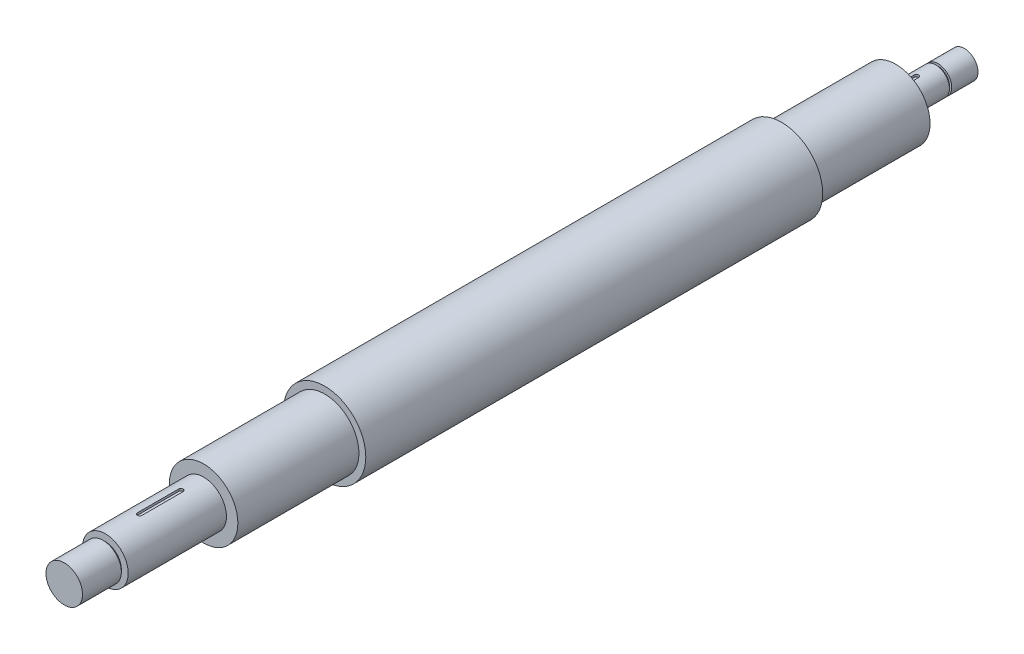
SolidWorks part; units mm, degrees
material "AISI 304"
ref_plane "Front Plane" through (0, 0, 0) normal (0, 0, 1) x (1, 0, 0)
ref_plane "Top Plane" through (0, 0, 0) normal (0, 1, 0) x (1, 0, 0)
ref_plane "Right Plane" through (0, 0, 0) normal (1, 0, 0) x (0, 0, -1)
sketch "Sketch1" plane through (0, 0, 0) normal (0, 0, 1) x (1, 0, 0)
  circle A0 centre (0, 0) radius 15
  dimension "D1" = 30
extrude "Boss-Extrude1" add sketch "Sketch1" along normal blind 50
sketch "Sketch2" plane through (0, 0, 50) normal (0, 0, 1) x (1, 0, 0)
  circle A0 centre (0, 0) radius 18
  dimension "D1" = 36
extrude "Boss-Extrude2" add sketch "Sketch2" along normal blind 200
sketch "Sketch3" plane through (0, 0, 250) normal (0, 0, 1) x (1, 0, 0)
  circle A0 centre (0, 0) radius 15
  dimension "D1" = 30
extrude "Boss-Extrude3" add sketch "Sketch3" along normal blind 53
sketch "Sketch4" plane through (0, 0, 0) normal (0, 0, -1) x (-1, 0, 0)
  circle A0 centre (0, 0) radius 6
  dimension "D1" = 12
extrude "Boss-Extrude4" add sketch "Sketch4" along normal blind 30
cosmetic thread "Cosmetic Thread1" parameters "D1"=11.4999, "D2"=11.5
sketch "Sketch5" plane through (0, 0, 0) normal (0, 1, 0) x (1, 0, 0)
  line L0 (0, 30) -> (0, -1.1912) construction
  line L1 (6, 30) -> (-6, 30) construction
  line L2 (15, 0) -> (-15, 0) construction
  line L3 (1, 9) -> (-1, 9)
  line L4 (1, 9) -> (1, 5)
  line L5 (1, 5) -> (-1, 5)
  line L6 (-1, 9) -> (-1, 5)
  line L7 (1, 9) -> (-1, 5) construction
  line L8 (1, 5) -> (-1, 9) construction
  circle A0 centre (0, 5) radius 1
  circle A1 centre (0, 9) radius 1
  point P7 (0, 7)
  point P16 (0, 5)
  dimension "D2" = 2
  dimension "D1" = 4
  dimension "D3" = 5
extrude "Cut-Extrude1" cut sketch "Sketch5" along normal blind 10 from offset 5 contours L3 A1 | L3 A1 | A1 L6 A0 L4 | L5 A0 | L5 A0
sketch "Sketch6" plane through (0, 0, -30) normal (0, 0, -1) x (-1, 0, 0)
  circle A0 centre (0, 0) radius 6
  circle A1 centre (0, 0) radius 5
  dimension "D1" = 10
extrude "Cut-Extrude3" cut sketch "Sketch6" against normal blind 1 from offset 11.5 offset against normal yes
sketch "Sketch7" plane through (0, 0, 303) normal (0, 0, 1) x (1, 0, 0)
  circle A0 centre (0, 0) radius 10
  dimension "D1" = 20
extrude "Boss-Extrude5" add sketch "Sketch7" along normal blind 43
sketch "Sketch9" plane through (0, 5, 0) normal (0, 1, 0) x (1, 0, 0)
  line L0 (0, -303) -> (0, -337.2251) construction
  line L1 (-10, -303) -> (10, -303) construction
  line L3 (-1, -313) -> (1, -313)
  line L4 (-1, -313) -> (-1, -331)
  line L5 (-1, -331) -> (1, -331)
  line L6 (1, -313) -> (1, -331)
  line L7 (-1, -313) -> (1, -331) construction
  line L8 (-1, -331) -> (1, -313) construction
  circle A0 centre (0, -313) radius 1
  circle A1 centre (0, -331) radius 1
  point P5 (0, -322)
  dimension "D1" = 2
  dimension "D2" = 18
  dimension "D3" = 10
extrude "Cut-Extrude4" cut sketch "Sketch9" along normal blind 12 from offset 4 contours A1 L6 A0 L4 | L5 A1 | L5 A1 | L3 A0 | L3 A0
sketch "Sketch8" plane through (0, 0, 346) normal (0, 0, 1) x (1, 0, 0)
  circle A0 centre (0, 0) radius 8
  dimension "D1" = 16
extrude "Boss-Extrude6" add sketch "Sketch8" along normal blind 18
cosmetic thread "Cosmetic Thread2" parameters "D1"=17, "D2"=15
sketch "Sketch10" plane through (0, 0, 364) normal (0, 0, 1) x (1, 0, 0)
  circle A0 centre (0, 0) radius 7
  circle A1 centre (0, 0) radius 9
  dimension "D1" = 14
  dimension "D2" = 18
extrude "Cut-Extrude6" cut sketch "Sketch10" along normal blind 1 from offset 18
